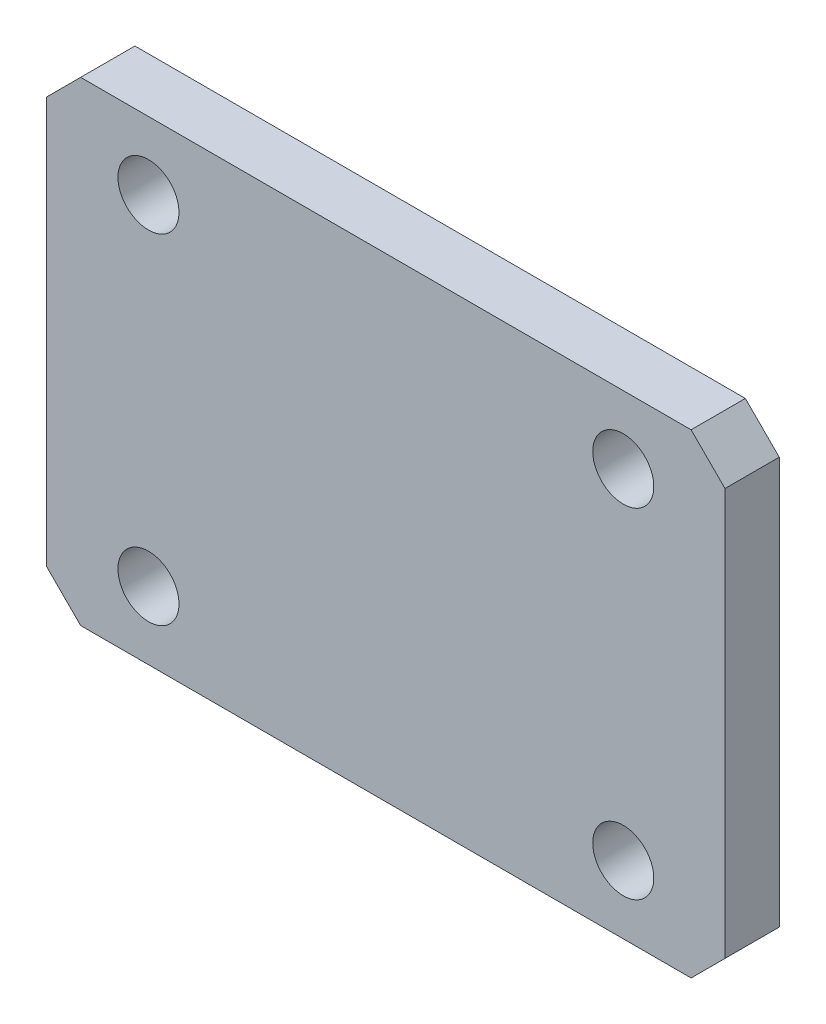
SolidWorks part; units mm, degrees
material "1023 碳钢板 (SS)"
ref_plane "Front Plane" through (0, 0, 0) normal (0, 0, 1) x (1, 0, 0)
ref_plane "Top Plane" through (0, 0, 0) normal (0, 1, 0) x (1, 0, 0)
ref_plane "Right Plane" through (0, 0, 0) normal (1, 0, 0) x (0, 0, -1)
ref_plane "Plane1" through (0, 0, -15) normal (0, 0, 1) x (1, 0, 0)
sketch "Sketch1" plane through (0, 0, -15) normal (0, 0, 1) x (1, 0, 0)
  line L0 (-11.8, -210) -> (11.8, -210) construction
  line L1 (-50, -140) -> (50, -140)
  line L2 (-50, -140) -> (-50, -210)
  line L3 (-50, -210) -> (50, -210)
  line L4 (50, -140) -> (50, -210)
  line L5 (-50, -140) -> (50, -210) construction
  line L6 (-50, -210) -> (50, -140) construction
  point P0 (0, -175)
  dimension "D1" = 100
  dimension "D2" = 70
  dimension "D3" = 0
extrude "Boss-Extrude1" add sketch "Sketch1" against normal blind 8
sketch "Sketch2" plane through (0, 0, -23) normal (0, 0, -1) x (-1, 0, 0)
  line L5 (-35, -150) -> (35, -200) construction
  line L6 (-35, -200) -> (35, -150) construction
  circle A0 centre (-35, -150) radius 4.5
  circle A1 centre (35, -150) radius 4.5
  circle A2 centre (35, -200) radius 4.5
  circle A3 centre (-35, -200) radius 4.5
  point P0 (0, -175)
extrude "Cut-Extrude1" cut sketch "Sketch2" against normal blind 8
chamfer "Chamfer1" distance 5 angle 45 4 edges at (-50, -140, -19) (-50, -210, -19) (50, -140, -19) (50, -210, -19)
